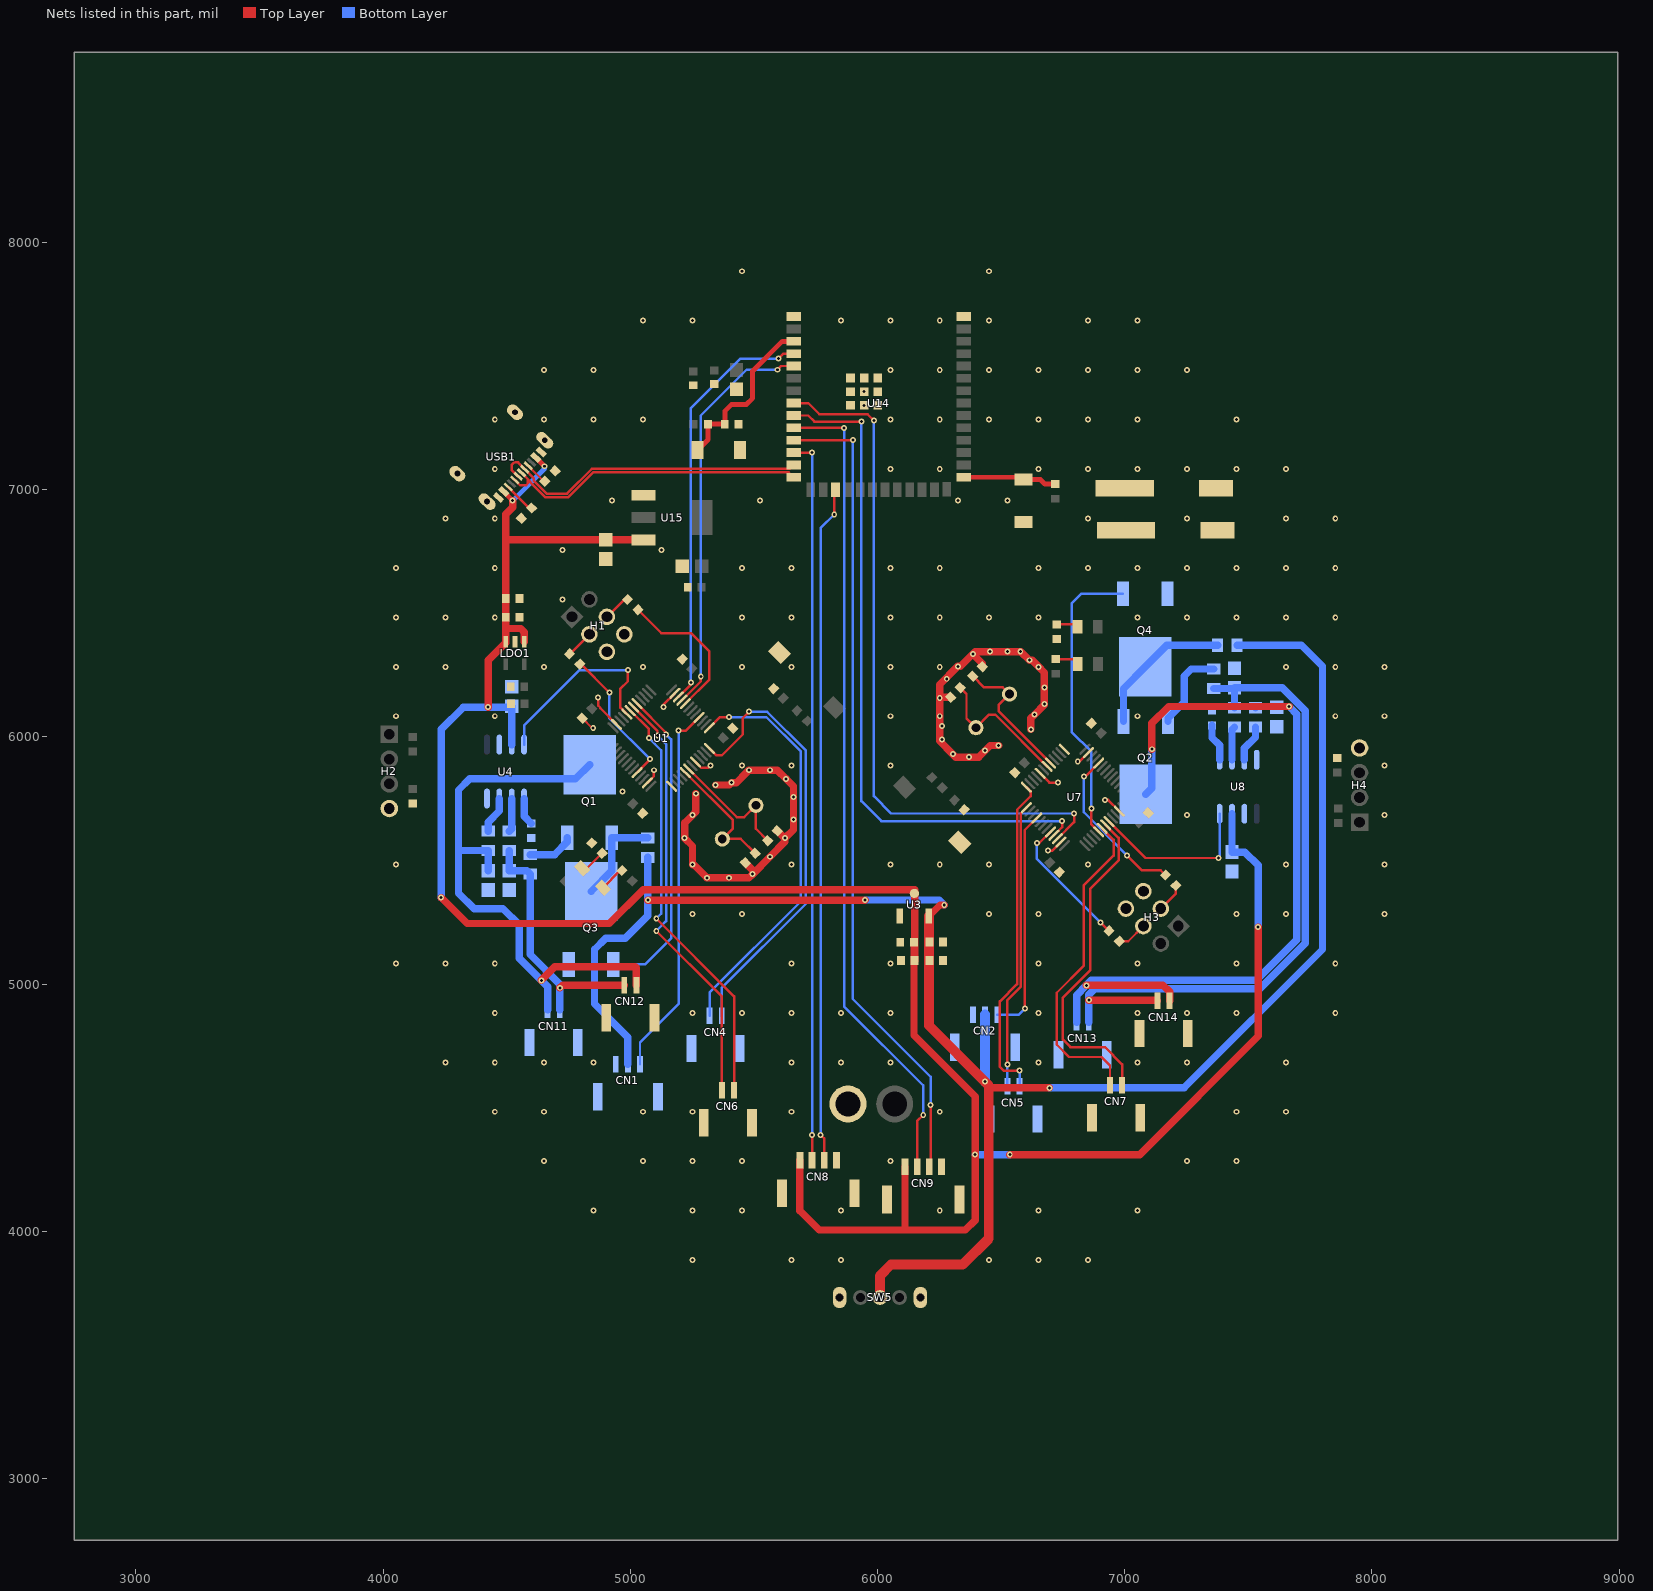
[diagram p0: the nets of this part, all layers, seen from the top]
# Altium PCB MISC62500.pcbdoc (part 2 of 3)
Units mil, origin at the board's own origin, x right, y up, seen from the top; angles counter-clockwise.
Board outline 6245 x 6020 mil, 2 copper layers (Top Layer, Bottom Layer), stack 62.206 mil thick; 106 components, 73 nets, 432 pads, 293 vias.

## Via types
v1: diameter 24, hole 12, Top Layer to Bottom Layer, 293 vias

## Nets (pads, with @x,y where several pads share a name; then routed paths per layer and width w, separated by ;. In a path a pad name is that pad's centre, name@x,y a point inside that pad or via, vN(x,y) a via of type N, cw(c..) or ccw(c..) an arc to the next point about the centre after c; other vN are vias at no path point)
$3N2273: PWR.2 R1.1 | length 105.8
  Top Layer w10: PWR.2@4805.05,5468.89 4825.84,5468.89 R1.1@4885.97,5529.03
$3N2332: PC13.2 R2.1 | length 105.6
  Top Layer w10: PC13.2@4889.24,5389.24 4959.03,5459.03 R2.1@4965.97,5459.03
$3N2745: H1.3 R3.2 | length 113.2
  Top Layer w10: R3.2@4754.03,6335.97 4755.97,6335.97 H1.3@4834.64,6414.64
$3N2755: H1.4 R4.1 | length 112.9
  Top Layer w10: H1.4@4905.36,6485.36 4975.97,6555.97 R4.1@4989.03,6555.97
$3N6906: R8.1 U4.7 | length 150.1
  Bottom Layer w30: R8.1@4425.26,5618.92 4425.26,5655.26 4470.26,5700.26 U4.7@4470.26,5750.4
$3N6912: R9.1 U4.6 | length 135.6
  Bottom Layer w30: R9.1@4510.26,5618.92 4520.26,5628.92 U4.6@4520.26,5750.4
$3N7100: Q1.3 R10.2 | length 188.1
  Bottom Layer w30: R10.2@4595.26,5523.92 4693.92,5523.92 4745.18,5575.18 Q1.3@4745.18,5592.11
$3N9265: PWR1.2 R11.1 | length 87.7
  Top Layer w10: R11.1@6725,6454.66 6798.99,6454.66 PWR1.2@6808.65,6445
$3N9268: PC14.2 R12.1 | length 96.8
  Top Layer w10: R12.1@6720.9,6314.62 6789.89,6314.62 PC14.2@6809.55,6294.96
$3N9271: H3.3 R13.2 | length 118.8
  Top Layer w10: H3.3@7146.26,5305.32 7206.88,5365.93 R13.2@7206.88,5398.99
$3N9274: H3.4 R14.1 | length 122.7
  Top Layer w10: R14.1@6978.22,5173.38 7014.33,5173.38 H3.4@7075.55,5234.61
$3N9413: R18.1 U8.7 | length 150.1
  Bottom Layer w30: U8.7@7483.98,5907.52 7483.98,5953.98 7528.98,5998.98 R18.1@7528.98,6039
$3N9417: R19.1 U8.6 | length 135.6
  Bottom Layer w30: U8.6@7433.98,5907.52 7433.98,6029 R19.1@7443.98,6039
$3N9436: Q2.3 R20.2 | length 341.6
  Bottom Layer w30: Q2.3@7175.08,6062.44 7175.08,6075.08 7240,6140 7240,6245 7269.37,6274.37 R20.2@7360,6274.37
$3N12622: R21.2 U4.5 | length 113.1
  Bottom Layer w30: U4.5@4570.26,5750.4 4570.26,5679.4 R21.2@4600,5649.66
$3N12763: R22.2 U8.5 | length 151.7
  Bottom Layer w30: R22.2@7353.16,6046.41 7353.16,5996.84 7383.98,5966.02 U8.5@7383.98,5907.52
$3N48437: Q1.1 Q3.2 R27.1 | length 398.6
  Bottom Layer w30: Q3.2@4841.15,5374.36 4925.34,5458.55 Q1.1@4925.34,5592.03 4926.16,5591.21 R27.1@5071.07,5591.21
$3N48829: Q2.1 Q4.2 R28.1 | length 585.9
  Bottom Layer w30: Q2.1@6994.92,6062.52 6994.92,6195.39 Q4.2@7083.08,6283.55 7169.53,6370 R28.1@7375.63,6370
$4N2238: R31.2 USB1.A5 | length 93.2
  Top Layer w10: USB1.A5@4586.85,7096.87 4649.69,7034.03 R31.2@4654.03,7034.03
$4N2242: R32.2 USB1.B5 | length 130.1
  Top Layer w10: USB1.B5@4506.01,7010.76 4590.8,6925.97 R32.2@4600.97,6925.97
+5V: C1.2 C2.2 C15.1 C17.1 C39.2 CN8.1 CN9.1 LDO1.1 LDO1.3 U2.1 U3.2 U4.3 U8.3 U9.1 U15.3 USB1.A4B9 USB1.B4A9 | length 10075.2
  Top Layer w20: USB1.B4A9@4488.49,6992.11 4488.49,6991.57 v1(4524.27,6955.79) ; USB1.A4B9@4617.84,7129.88 v1(4653.1,7094.63)
  Top Layer w30: v1(4235,5350) 4340,5245 4915,5245 5051.97,5381.97 6149.05,5381.97 6149.87,5381.15 C17.1@6149.87,5094.82 ; v1(4425,6120) 4425,6310 4496.28,6381.28 LDO1.3@4496.28,6384.65 4496.28,6438.19 ; v1(4524.27,6955.79) 4524.27,6929.27 4496.28,6901.28 4496.28,6806.28 ; LDO1.1@4571.08,6384.65 4571.08,6423.92 4556.81,6438.19 4496.28,6438.19 ; U15.3@5053.04,6796.55 5051.7,6797.89 C39.2@4900.52,6797.89 4504.67,6797.89 4496.28,6806.28 ; CN8.1@5686.18,4286.63 5686.18,4083.82 5765,4005 6106.18,4005 ; CN9.1@6111.18,4261.63 6111.18,4010 6106.18,4005 ; C15.1@6147.46,5168.7 6147.46,4792.54 6395,4545 v1(6395,4310) 6395,4045 6355,4005 6106.18,4005 ; v1(6535,4310) 7060,4310 7540,4790 v1(7540,5230) ; 4496.28,6438.19 4496.28,6806.28
  Bottom Layer w20: v1(4524.27,6955.79) 4653.1,7084.63 v1(4653.1,7094.63)
  Bottom Layer w30: v1(4235,5350) 4235,6030 4325,6120 v1(4425,6120) 4516.34,6120 U2.1@4520.26,6123.92 U4.3@4520.26,5968.7 ; v1(6395,4310) v1(6535,4310) ; U8.3@7433.98,5689.22 U9.1@7433.98,5534 7486,5534 7540,5480 v1(7540,5230)
BOOT0: R3.1 U1.44 | length 580.5
  Top Layer w10: R3.1@4795.97,6294.03 4800.97,6294.03 v1(4915,6180) ; U1.44@5027.57,5855.81 5080,5908.24 v1(5080,5910)
  Bottom Layer w10: v1(4915,6180) 4915,6075 v1(5080,5910)
BOOT0B: R13.1 U7.44 | length 662.3
  Top Layer w10: v1(6835,5840) 6840.58,5840 U7.44@6894.73,5894.16 ; v1(7010,5520) 7070,5460 7145.87,5460 R13.1@7164.93,5440.93
  Bottom Layer w10: v1(6835,5840) 6835,5695 v1(7010,5520)
BOOT1: R4.2 U1.20 | length 610.3
  Top Layer w10: R4.2@5030.97,6514.03 5125,6420 5245,6420 5320,6345 5320,6231.76 U1.20@5222.43,6134.19
BOOT1B: R14.2 U7.20 | length 549.1
  Top Layer w10: v1(6645,5570) 6654.1,5570 U7.20@6699.87,5615.77 ; v1(6901.84,5249.76) R14.2@6936.27,5215.33
  Bottom Layer w10: v1(6645,5570) 6645,5506.6 v1(6901.84,5249.76)
CANH: C18.2 CN11.2 CN12.2 Q1.2 R8.2 | length 2359.7
  Top Layer w30: v1(4640,5015) 4695,5070 5020,5070 5024.61,5065.39 CN12.2@5024.61,4995.94
  Bottom Layer w30: C18.2@4425.26,5458.92 R8.2@4425.26,5540.18 4305,5540.18 ; CN11.2@4665.39,4895.94 4665.39,4989.61 v1(4640,5015) 4550,5105 4550,5240 4485,5305 4368.06,5305 4305,5368.06 4305,5540.18 ; Q1.2@4835.34,5887.07 4778.27,5830 4350,5830 4305,5785 4305,5540.18
CANHB: C33.2 CN13.2 CN14.2 Q2.2 R18.2 | length 3452.5
  Top Layer w30: v1(6845,4995) 7155,4995 7181.59,4968.41 CN14.2@7181.59,4931.77 ; v1(7110,5950) 7110,6055 7177.74,6122.74 v1(7665,6122.74)
  Bottom Layer w30: CN13.2@6805.39,4845.94 6805.39,4955.39 v1(6845,4995) 6865,5015 7531.92,5015 7696,5179.08 7696,6091.74 v1(7665,6122.74) 7533.98,6122.74 R18.2@7528.98,6117.74 ; Q2.2@7084.92,5767.48 7110,5792.56 v1(7110,5950)
CANL: C19.2 CN11.1 CN12.1 R9.2 R10.1 | length 1035.9
  Top Layer w30: v1(4715,4985) 4725.94,4995.94 CN12.1@4975.4,4995.94
  Bottom Layer w30: R9.2@4510.26,5540.18 C19.2@4510.26,5458.92 4581.52,5458.92 R10.1@4595.26,5445.18 4595.26,5119.74 4715,5000 v1(4715,4985) 4715,4896.34 CN11.1@4714.6,4895.94
CANLB: C34.2 CN13.1 CN14.1 R19.2 R20.1 | length 2783.1
  Top Layer w30: v1(6855,4935) 7129.14,4935 CN14.1@7132.37,4931.77
  Bottom Layer w30: CN13.1@6854.6,4845.94 6854.6,4934.6 v1(6855,4935) 6855,4956.92 6879.08,4981 7546,4981 7730,5165 7730,6105.82 7636.82,6199 C34.2@7443.98,6199 ; R20.1@7360,6195.63 7440.61,6195.63 C34.2@7443.98,6199 ; R19.2@7443.98,6117.74 C34.2@7443.98,6199
EN: C38.2 R29.2 SW3.2 U14.3 | length 702.5
  Top Layer w20: SW3.2@5271.94,7160 5314.66,7202.72 R29.2@5314.66,7265 C38.2@5382.44,7265 5382.44,7317.44 5410,7345 5470,7345 5495,7370 5495,7480 5615.19,7600.19 U14.3@5660.51,7600.19
GND: C1.1 C2.1 C3.1 C4.1 C5.1 C6.1 C7.1 C8.1 C9.1 C10.2 C11.2 C14.1 C15.2 C16.1 C17.2 C18.1 C19.1 C24.1 C25.1 C26.1 C27.1 C28.1 C29.2 C30.2 C33.1 C34.1 C35.1 C36.1 C37.1 C38.1 C39.1 C40.1 C41.2 CN1.3 CN1.4 CN1.5 CN2.3 CN2.4 CN2.5 CN3.1 CN3.2 CN4.3 CN4.4 CN5.3 CN5.4 CN6.3 CN6.4 CN7.3 CN7.4 CN8.4 CN8.5 CN8.6 CN9.4 CN9.5 CN9.6 CN10.1 CN10.2 CN11.3 CN11.4 CN12.3 CN12.4 CN13.3 CN13.4 CN14.3 CN14.4 H1.5 H1.6 H2.4 H3.5 H3.6 H4.4 LDO1.2 Q3.3 Q4.3 R1.2 R6.1 R11.2 R16.1 R21.1 R22.1 R31.1 R32.1 SW1.2 SW2.2 SW3.1 SW4.1 SW5.4 SW5.5 U1.1 U1.8 U1.23 U1.35 U1.47 U2.2 U3.1 U4.2 U4.8 U6.1 U7.1 U7.8 U7.23 U7.35 U7.47 U8.2 U8.8 U9.2 U14.1 U14.40 U14.41 U15.1 USB1.13 USB1.14 USB1.A1B12 USB1.B1A12 | length 3571.6
  Top Layer w10: C7.1@4805.51,6075.51 4846.02,6035 v1(4850,6035) ; v1(4870,6160) 4870,6126.8 4879.15,6117.65 4879.15,6115.58 U1.35@4944.05,6050.68 ; U1.47@5069.32,5814.05 5095,5839.73 v1(5095,5865) ; v1(5135,6120) 5135,6130.27 U1.23@5180.68,6175.95 ; U1.8@5264.19,5897.57 5286.76,5875 5315,5875 v1(5325,5885) ; U7.8@6658.11,5852.39 6695.5,5815 v1(6730,5815) ; v1(6690,5540) 6707.61,5540 U7.23@6741.62,5574.01 ; v1(6810,5900) 6817.07,5900 U7.47@6852.98,5935.91 ; v1(6920,5745) 6932.53,5745 U7.35@6978.25,5699.28
  Top Layer w30: v1(5265,5770) 5265,5696.75 v1(5251.71,5683.46) 5220,5651.75 v1(5220,5590) 5251.71,5558.29 v1(5251.71,5483.46) 5256.54,5483.46 v1(5310,5430) v1(5398.89,5430) 5480,5430 v1(5495,5445) ; v1(5345,5805.38) 5400.38,5805.38 v1(5410,5815) 5429.33,5815 5471.07,5856.74 ccw(c5451.71,5883.46) 5478.44,5864.11 v1(5479.33,5865) ; C10.2@5465.51,5490.51 5495,5461.02 v1(5495,5445) ; v1@5479.92,5865 v1(5565,5865) 5595,5865 v1(5630,5830) 5660,5800 v1(5660,5756.52) v1(5660,5665) 5660,5625 v1(5625,5590) ; C11.2@5594.49,5619.49 5595.51,5619.49 v1(5625,5590) ; C30.2@6295.51,6160.51 6255.43,6160.51 v1(6251.71,6156.8) ; C29.2@6424.49,6284.49 6424.49,6296.12 v1(6385.61,6335) ; v1(6490,5965) 6455.67,5965 v1(6435.56,5944.89) 6408.69,5918.02 v1(6370.7,5918.02) 6316.98,5918.02 v1(6305,5930) 6251.71,5983.29 v1(6251.71,6083.46) v1(6251.71,6156.8) ; v1(6620,6030) 6620,6075 v1(6635,6090) 6674.8,6129.8 v1(6674.8,6133.63) v1(6674.8,6200) 6674.8,6260.38 v1(6651.71,6283.46) 6625.17,6310 v1(6615,6310) 6580,6345 v1(6577.47,6345) v1(6526.5,6345) v1(6455,6345) 6395.61,6345 v1(6385.61,6335) ; v1(5495,5445) v1(5565,5515) 5625,5575 v1(5625,5590) ; v1(6251.71,6156.8) 6251.71,6211.71 v1(6325,6285) 6335.61,6285 v1(6385.61,6335)
  other v1: 5251.71,3883.46 5651.71,3883.46 5851.71,3883.46 6451.71,3883.46 6651.71,3883.46 6851.71,3883.46 4851.71,4083.46 5251.71,4083.46 5451.71,4083.46 5851.71,4083.46 6251.71,4083.46 6651.71,4083.46 7051.71,4083.46 4651.71,4283.46 5051.71,4283.46 5251.71,4283.46 5451.71,4283.46 6051.71,4283.46 7251.71,4283.46 7451.71,4283.46 4451.71,4483.46 4651.71,4483.46 5051.71,4483.46 5251.71,4483.46 5651.71,4483.46 6251.71,4483.46 7451.71,4483.46 7651.71,4483.46 4251.71,4683.46 4451.71,4683.46 4651.71,4683.46 4851.71,4683.46 5651.71,4683.46 5851.71,4683.46 6051.71,4683.46 6651.71,4683.46 7051.71,4683.46 7251.71,4683.46 7651.71,4683.46 4451.71,4883.46 5251.71,4883.46 5451.71,4883.46 5651.71,4883.46 5851.71,4883.46 6051.71,4883.46 6651.71,4883.46 7051.71,4883.46 7251.71,4883.46 7451.71,4883.46 7851.71,4883.46 4051.71,5083.46 4251.71,5083.46 4451.71,5083.46 5651.71,5083.46 6051.71,5083.46 6651.71,5083.46 7051.71,5083.46 7451.71,5083.46 7851.71,5083.46 5251.71,5283.46 5451.71,5283.46 6451.71,5283.46 6651.71,5283.46 7451.71,5283.46 7651.71,5283.46 8051.71,5283.46 4051.71,5483.46 5651.71,5483.46 6051.71,5483.46 6251.71,5483.46 6451.71,5483.46 6851.71,5483.46 7651.71,5483.46 8051.71,5483.46 7251.71,5683.46 8051.71,5683.46 4969.1,5779.1 5451.71,5883.46 5651.71,5883.46 6051.71,5883.46 8051.71,5883.46 6260,5990 6260,6044.64 4051.71,6083.46 4451.71,6083.46 6051.71,6083.46 7051.71,6083.46 7851.71,6083.46 8051.71,6083.46 6280,6235 4051.71,6283.46 4251.71,6283.46 4651.71,6283.46 5051.71,6283.46 5451.71,6283.46 5651.71,6283.46 6051.71,6283.46 6251.71,6283.46 7651.71,6283.46 7851.71,6283.46 8051.71,6283.46 4051.71,6483.46 4251.71,6483.46 4451.71,6483.46 5451.71,6483.46 5651.71,6483.46 6051.71,6483.46 6251.71,6483.46 6451.71,6483.46 6651.71,6483.46 7051.71,6483.46 7251.71,6483.46 7451.71,6483.46 7651.71,6483.46 7851.71,6483.46 4725.38,6556.22 4051.71,6683.46 4451.71,6683.46 5451.71,6683.46 5651.71,6683.46 6051.71,6683.46 6251.71,6683.46 6651.71,6683.46 6851.71,6683.46 7051.71,6683.46 7251.71,6683.46 7451.71,6683.46 7651.71,6683.46 7851.71,6683.46 4725.38,6756.22 5125.38,6756.22 4251.71,6883.46 4451.71,6883.46 6851.71,6883.46 7251.71,6883.46 7651.71,6883.46 7851.71,6883.46 4925.38,6956.22 5525.38,6956.22 6325.38,6956.22 6525.38,6956.22 4451.71,7083.46 6051.71,7083.46 6251.71,7083.46 6651.71,7083.46 6851.71,7083.46 7051.71,7083.46 7251.71,7083.46 7451.71,7083.46 7651.71,7083.46 4451.71,7283.46 4651.71,7283.46 4851.71,7283.46 5051.71,7283.46 6051.71,7283.46 6251.71,7283.46 6451.71,7283.46 6651.71,7283.46 6851.71,7283.46 7051.71,7283.46 7451.71,7283.46 5945.94,7341.14 5945.94,7396.26 4651.71,7483.46 4851.71,7483.46 6051.71,7483.46 6251.71,7483.46 6451.71,7483.46 6651.71,7483.46 6851.71,7483.46 7051.71,7483.46 7251.71,7483.46 5051.71,7683.46 5251.71,7683.46 5851.71,7683.46 6051.71,7683.46 6251.71,7683.46 6451.71,7683.46 6851.71,7683.46 7051.71,7683.46 5451.71,7883.46 6451.71,7883.46
IO0: R30.2 SW4.2 U14.27 | length 381.6
  Top Layer w20: U14.27@6349.49,7050.19 6580.82,7050.19 SW4.2@6590,7041.02 6658.98,7041.02 6677.67,7022.33 R30.2@6719.59,7022.33
IO4: U1.22 U14.4 | length 1695.6
  Top Layer w10: U1.22@5194.59,6162.03 5245,6212.44 v1(5245,6220) ; v1(5600,7530) 5620.19,7550.19 U14.4@5660.51,7550.19
  Bottom Layer w10: v1(5245,6220) 5245,7330 5445,7530 v1(5600,7530)
IO5: U1.21 U14.5 | length 1642
  Top Layer w10: U1.21@5208.52,6148.11 5285,6224.59 v1(5285,6245) ; v1(5595,7485) 5610.19,7500.19 U14.5@5660.51,7500.19
  Bottom Layer w10: v1(5285,6245) 5285,7300 5470,7485 v1(5595,7485)
IO8: CN8.2 U14.12 | length 2938.3
  Top Layer w10: U14.12@5660.51,7150.19 5660.7,7150 v1(5735.39,7150) ; CN8.2@5735.39,4286.63 v1(5735.39,4390)
  Bottom Layer w10: v1(5735.39,4390) v1(5735.39,7150)
IO9: CN8.3 U14.17 | length 2744.1
  Top Layer w10: v1(5770,4390) 5784.6,4375.4 CN8.3@5784.6,4286.63 ; v1(5825,6900) 5825,6994.81 U14.17@5830,6999.81
  Bottom Layer w10: v1(5770,4390) 5770,6845 v1(5825,6900)
IO15: U7.22 U14.8 | length 2842.5
  Top Layer w10: U14.8@5660.51,7350.19 5719.81,7350.19 5765,7305 5960,7305 v1(5985,7280) ; U7.22@6727.71,5587.93 6795,5655.22 v1(6795,5690)
  Bottom Layer w10: v1(5985,7280) 5985,5760 6055,5690 v1(6795,5690)
IO16: U7.21 U14.9 | length 2735.9
  Top Layer w10: U14.9@5660.51,7300.19 5660.7,7300 5720,7300 5745,7275 v1(5935,7275) ; U7.21@6713.79,5601.85 6746.43,5634.5 v1(6746.43,5659.5)
  Bottom Layer w10: v1(5935,7275) 5935,5740 6015.5,5659.5 v1(6746.43,5659.5)
IO17: CN9.2 U14.10 | length 3335.7
  Top Layer w10: U14.10@5660.51,7250.19 5660.7,7250 v1(5865,7250) ; CN9.2@6160.39,4261.63 6160.39,4445.39 v1(6185,4470)
  Bottom Layer w10: v1(5865,7250) 5865,4910 6185,4590 v1(6185,4470)
IO18: CN9.3 U14.11 | length 3310.7
  Top Layer w10: U14.11@5660.51,7200.19 5660.7,7200 v1(5900,7200) ; CN9.3@6209.6,4261.63 6215,4267.03 v1(6215,4510)
  Bottom Layer w10: v1(5900,7200) 5900,4940 6215,4625 v1(6215,4510)
IO19: U14.13 USB1.A7 USB1.B7 | length 1308.6
  Top Layer w10: USB1.A7@4546.43,7053.82 4546.18,7053.82 4520,7080 4520,7100 4530,7110 4545.9,7110 USB1.B7@4573.38,7082.53 4610,7045.9 4610,7035 4661,6984 4744,6984 4844,7084 5644.31,7084 U14.13@5660.51,7100.19
IO20: U14.14 USB1.A6 USB1.B6 | length 1274.9
  Top Layer w10: USB1.B6@4532.96,7039.47 4554.94,7017.5 4577.5,7017.5 4585,7025 4585,7043.09 ; USB1.A6@4559.91,7068.18 4585,7043.09 ; U14.14@5660.51,7050.19 5640.7,7070 4849.8,7070 4749.8,6970 4655.2,6970 4596,7029.2 4596,7032.09 4585,7043.09
OSCIN: C10.1 U1.5 Y2.1 | length 522.5
  Top Layer w10: U1.5@5222.43,5855.81 5415,5663.24 5415,5630 Y2.1@5372.07,5587.07 5446.9,5587.08 C10.1@5504.49,5529.49
OSCINB: C29.1 U7.5 Y3.1 | length 562.2
  Top Layer w10: C29.1@6385.51,6245.51 6431.02,6200 6506.71,6200 Y3.1@6533.83,6172.89 6490,6129.06 6490,6104.03 U7.5@6699.87,5894.16
OSOUT: C11.1 U1.6 Y2.2 | length 534.2
  Top Layer w10: U1.6@5236.36,5869.73 5431.08,5675 5460,5675 Y2.2@5507.93,5722.93 5507.92,5628.1 C11.1@5555.51,5580.51
OSOUTB: C30.1 U7.6 Y3.2 | length 585.5
  Top Layer w10: C30.1@6334.49,6199.49 6360,6173.98 6360,6075.02 Y3.2@6397.98,6037.03 6450.94,6090 6476.18,6090 U7.6@6685.95,5880.23
OUTPUT: C14.2 C16.2 CN1.2 CN2.2 R27.2 R28.2 SW5.2 U3.3 | length 7695.7
  Top Layer w30: v1(5071.07,5339.39) 5949.39,5339.39 v1(5950,5340) ; U3.3@6208.11,5275.18 6252.93,5320 v1(6270,5320) ; 6450,4590 6460,4580 v1(6695,4580)
  Top Layer w40: SW5.2@6010,3732.22 6010,3820 6055,3865 6345,3865 6450,3970 6450,4590 v1(6434.99,4605) 6208.11,4831.89 U3.3@6208.11,5275.18
  Bottom Layer w30: CN1.2@4989.99,4675.94 4989.99,4785.01 4855,4920 4855,5140 4900,5185 4980,5185 5071.07,5276.07 v1(5071.07,5339.39) R27.2@5071.07,5512.47 ; v1(5950,5340) 6250,5340 v1(6270,5320) ; v1(6695,4580) 7240,4580 7800,5140 7800,6285 7715,6370 R28.2@7454.37,6370
  Bottom Layer w40: v1(6434.99,4605) CN2.2@6434.99,4876.77
PA2: CN4.1 U1.12 | length 1793.1
  Top Layer w10: U1.12@5319.87,5953.25 5348.12,5925 5370,5925 5455,6010 5455,6076 v1@5480,6101
  Bottom Layer w10: CN4.1@5369.6,4870.94 5369.6,4984.6 5710,5325 5710,5945 5554,6101 v1@5480,6101
  other v1: 5480,6103
PA2B: CN5.1 U7.12 | length 1341.2
  Top Layer w10: v1(6575,4650) 6510,4650 6495,4665 6495,4930 6565,5000 6565,5705 6620,5760 6620,5779.15 U7.12@6602.43,5796.72
  Bottom Layer w10: CN5.1@6574.6,4585.94 6574.6,4649.6 v1(6575,4650)
PA3: CN4.2 U1.13 | length 1668.2
  Top Layer w10: U1.13@5319.87,6036.75 5363.12,6080 v1(5400,6080)
  Bottom Layer w10: CN4.2@5320.39,4870.94 5320.39,4965.39 5690,5335 5690,5940 5550,6080 v1(5400,6080)
PA3B: CN5.2 U7.13 | length 1159.2
  Top Layer w10: v1(6525.39,4675) 6525.39,4935.39 6580,4990 6580,5690.78 U7.13@6602.43,5713.21
  Bottom Layer w10: CN5.2@6525.39,4585.94 v1(6525.39,4675)
PA6: CN1.1 U1.16 | length 1518.9
  Top Layer w10: v1(5195,6025) 5224.59,6025 U1.16@5278.11,6078.52
  Bottom Layer w10: CN1.1@5039.21,4675.94 5039.21,4764.21 5195,4920 v1(5195,6025)
PA6B: CN2.1 U7.16 | length 913.2
  Top Layer w10: v1(6596.11,4901.11) 6595,4902.23 6595,5622.25 U7.16@6644.19,5671.45
  Bottom Layer w10: CN2.1@6484.21,4876.77 6571.77,4876.77 v1(6596.11,4901.11)
PA8: Q3.1 U1.29 | length 1283.7
  Top Layer w10: U1.29@5027.57,6134.19 5145,6016.76 v1(5145,6010)
  Bottom Layer w10: Q3.1@4931.15,5079.32 5059.32,5079.32 5165,5185 5165,5990 v1(5145,6010)
PA8B: Q4.1 U7.29 | length 1193.8
  Top Layer w10: v1(6865,5710) 6865,5645.5 U7.29@6894.73,5615.77
  Bottom Layer w10: v1(6865,5710) 6865,5940 6785,6020 6785,6540 6823.59,6578.59 Q4.1@6993.08,6578.59
PA9: CN6.1 U1.30 | length 1730.2
  Top Layer w10: U1.30@5013.64,6120.27 5110,6023.92 v1(5110,6005) ; v1(5105,5215) 5370.4,4949.6 CN6.1@5370.4,4570.94
  Bottom Layer w10: v1(5105,5215) 5145,5255 5145,5970 v1(5110,6005)
PA9B: CN7.1 U7.30 | length 1319.1
  Top Layer w10: U7.30@6908.66,5629.69 6955,5583.35 6955,5520 6835,5400 6835,5075 6725,4965 6725,4755 6775,4705 6905.83,4705 6940.4,4670.44 CN7.1@6940.4,4590.94
PA10: CN6.2 U1.31 | length 1725.9
  Top Layer w10: U1.31@4999.73,6106.36 5075,6031.08 v1(5075,5995) ; v1(5105,5265) 5419.61,4950.39 CN6.2@5419.61,4570.94
  Bottom Layer w10: v1(5075,5995) 5125,5945 5125,5285 v1(5105,5265)
PA10B: CN7.2 U7.31 | length 1348.5
  Top Layer w10: U7.31@6922.57,5643.61 6975,5591.18 6975,5500 6860,5385 6860,5055 6750,4945 6750,4775 6780,4745 6919.44,4745 6989.61,4674.82 CN7.2@6989.61,4590.94
PA11: U1.32 U4.4 | length 790.1
  Top Layer w10: U1.32@4985.81,6092.43 4960,6118.24 4960,6195 4990,6225 v1(4990,6270)
  Bottom Layer w10: U4.4@4570.26,5968.7 4570.26,6045.26 4795,6270 v1(4990,6270)
PA11B: U7.32 U8.4 | length 685.5
  Top Layer w10: U7.32@6936.5,5657.53 7084.03,5510 v1(7380,5510)
  Bottom Layer w10: v1(7380,5510) 7383.98,5513.98 U8.4@7383.98,5689.22